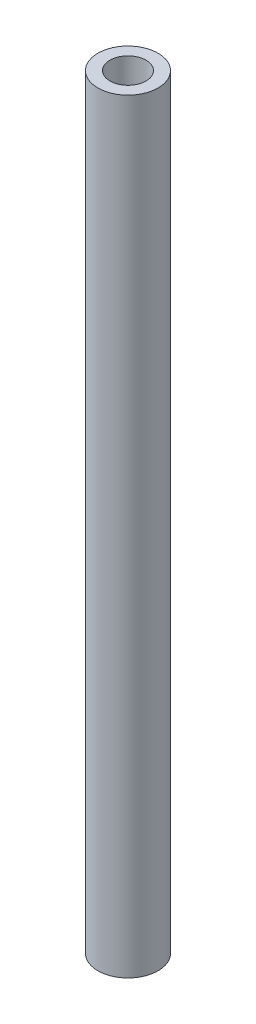
from build123d import *

# Parameters (mm, degrees)
SKETCH1_R           = 2.5
SKETCH1_R_2         = 1.5
BOSS_EXTRUDE1_DEPTH = 63.5
SKETCH2_R           = 1.5
SKETCH2_R_2         = 0.5
BOSS_EXTRUDE2_DEPTH = 2


with BuildPart() as part:
    # Sketch1 → Boss-Extrude1 (new body)
    with BuildSketch(Plane(origin=(0, 0, 0), x_dir=(1, 0, 0), z_dir=(0, 1, 0))):
        with Locations(Location((0, 0, 0), (0, 0, 270))):
            Circle(SKETCH1_R)
        with Locations(Location((0, 0, 0), (0, 0, 270))):
            Circle(SKETCH1_R_2, mode=Mode.SUBTRACT)
    extrude(amount=BOSS_EXTRUDE1_DEPTH)

    # Sketch2 → Boss-Extrude2 (add)
    with BuildSketch(Plane.XZ):
        with Locations(Location((0, 0, 0), (0, 0, 270))):
            Circle(SKETCH2_R)
        with Locations(Location((0, 0, 0), (0, 0, 270))):
            Circle(SKETCH2_R_2, mode=Mode.SUBTRACT)
    extrude(amount=-BOSS_EXTRUDE2_DEPTH)


solid = part.part
